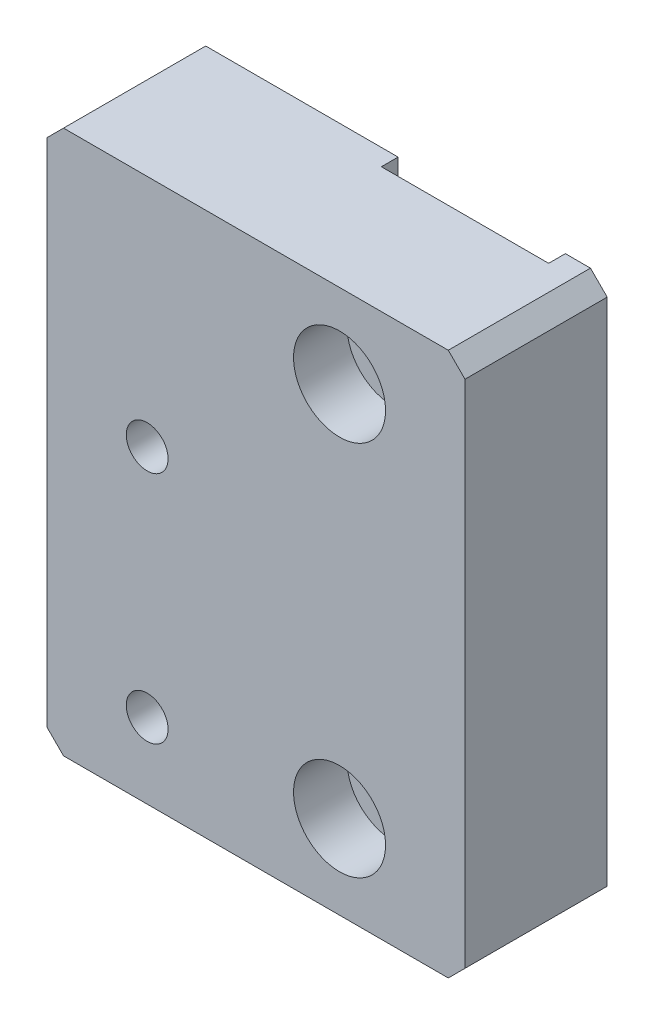
from build123d import *

# Parameters (mm, degrees)
SKETCH_2_W                     = 50
SKETCH_2_H                     = 65
EXTRUDE_1_DEPTH                = 17
SKETCH_3_W                     = 20
SKETCH_3_H                     = 2
CUT_EXTRUDE_1_DEPTH            = 84.749626865
CHAMFER_1_SIZE                 = 2
HOLE_WIZARD_M6_1_D             = 5
HOLE_WIZARD_M6_1_DEPTH         = 17
HOLE_WIZARD_M6_1_TIP           = 1.502151548
HOLE_WIZARD_M6_1_2_D           = 6.6
HOLE_WIZARD_M6_1_2_DEPTH       = 17
HOLE_WIZARD_M6_1_2_CBORE_D     = 11
HOLE_WIZARD_M6_1_2_CBORE_DEPTH = 6.4
HOLE_WIZARD_M6_1_2_TIP         = 1.982840043


with BuildPart() as part:
    # 草图2 → 凸台-拉伸1 (new body)
    with BuildSketch(Plane.XY):
        with Locations((25, -32.5)):
            Rectangle(SKETCH_2_W, SKETCH_2_H)
    extrude(amount=EXTRUDE_1_DEPTH)

    # 草图3 → 切除-拉伸1 (cut, through all)
    with BuildSketch(Plane.XZ.offset(65)):
        with Locations((35, 1)):
            Rectangle(SKETCH_3_W, SKETCH_3_H)
    extrude(amount=-CUT_EXTRUDE_1_DEPTH, mode=Mode.SUBTRACT)

    # 倒角1
    chamfer_1_edges = [part.edges().sort_by_distance(p)[0] for p in [
        (0, 0, 8.5),
        (50, 0, 8.5),
        (50, -65, 8.5),
        (0, -65, 8.5),
    ]]
    chamfer(chamfer_1_edges, length=CHAMFER_1_SIZE)

    # Hole Wizard M6 _1
    with Locations(Plane.XY.offset(17)):
        with Locations((12, -28), (12, -56)):
            Hole(HOLE_WIZARD_M6_1_D / 2, depth=HOLE_WIZARD_M6_1_DEPTH)
            with Locations((0, 0, -(HOLE_WIZARD_M6_1_DEPTH + HOLE_WIZARD_M6_1_TIP / 2))):  # 118° drill point
                Cone(0, HOLE_WIZARD_M6_1_D / 2, HOLE_WIZARD_M6_1_TIP, mode=Mode.SUBTRACT)

    # Hole Wizard M6 _1 2
    with Locations(Plane.XY.offset(17)):
        with Locations((35, -10), (35, -55)):
            CounterBoreHole(HOLE_WIZARD_M6_1_2_D / 2, HOLE_WIZARD_M6_1_2_CBORE_D / 2, HOLE_WIZARD_M6_1_2_CBORE_DEPTH, depth=HOLE_WIZARD_M6_1_2_DEPTH)
            with Locations((0, 0, -(HOLE_WIZARD_M6_1_2_DEPTH + HOLE_WIZARD_M6_1_2_TIP / 2))):  # 118° drill point
                Cone(0, HOLE_WIZARD_M6_1_2_D / 2, HOLE_WIZARD_M6_1_2_TIP, mode=Mode.SUBTRACT)


solid = part.part
